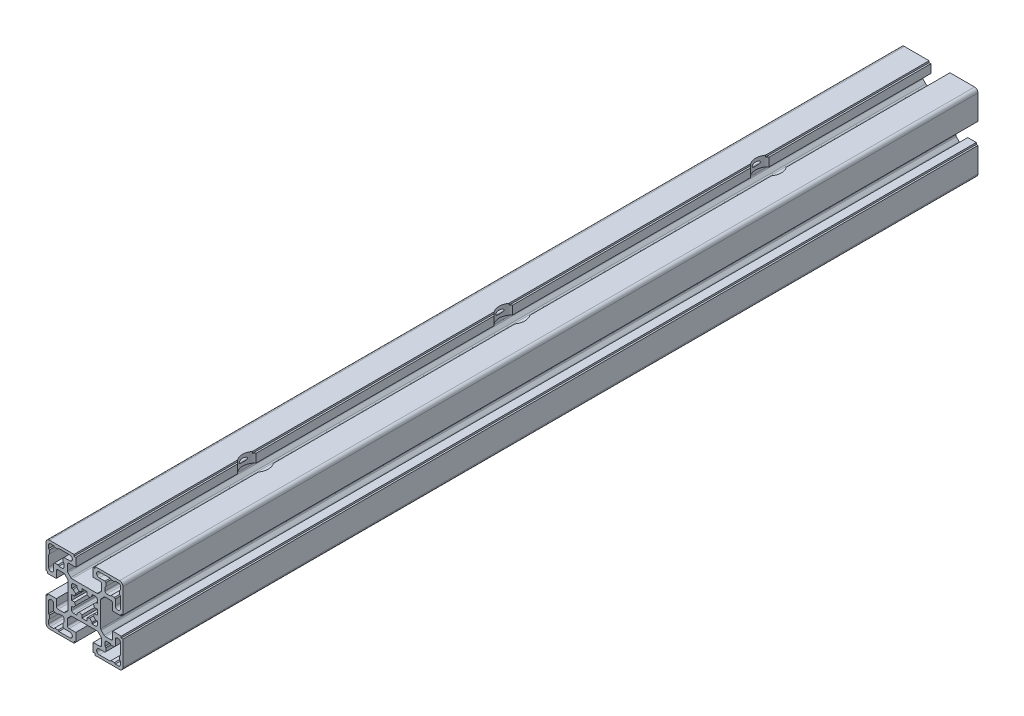
from build123d import *

# Parameters (mm, degrees)
EXTRUDE_1_DEPTH           = 500
HOLE_WIZARD_1_D           = 10
HOLE_WIZARD_1_CBORE_D     = 15
HOLE_WIZARD_1_CBORE_DEPTH = 9


with BuildPart() as part:
    # 草图1 → 拉伸1 (new body)
    with BuildSketch(Plane.XY):
        with BuildLine():
            Line((33.706586033, 40.501982097), (35.388566549, 38.820001582))
            ThreePointArc((35.388566549, 38.820001582), (35.712989897, 38.603228831), (36.09567333, 38.527108363))
            Line((36.09567333, 38.527108363), (39.413692815, 38.527108363))
            ThreePointArc((39.413692815, 38.527108363), (40.120799596, 38.820001582), (40.413692815, 39.527108363))
            Line((40.413692815, 39.527108363), (40.413692815, 43.427108363))
            Line((40.413692815, 43.427108363), (45.413692815, 43.427108363))
            Line((45.413692815, 43.427108363), (45.413692815, 42.427108363))
            Line((45.413692815, 42.427108363), (46.413692815, 42.427108363))
            Line((46.413692815, 42.427108363), (46.413692815, 28.027108363))
            ThreePointArc((46.413692815, 28.027108363), (45.827906377, 26.612894801), (44.413692815, 26.027108363))
            Line((44.413692815, 26.027108363), (30.013692814, 26.027108363))
            Line((30.013692814, 26.027108363), (30.013692814, 27.027108363))
            Line((30.013692814, 27.027108363), (29.013692814, 27.027108363))
            Line((29.013692814, 27.027108363), (29.013692814, 32.027108363))
            Line((29.013692814, 32.027108363), (32.913692814, 32.027108363))
            ThreePointArc((32.913692814, 32.027108363), (33.620799596, 32.320001582), (33.913692814, 33.027108363))
            Line((33.913692814, 33.027108363), (33.913692814, 36.345127848))
            ThreePointArc((33.913692814, 36.345127848), (33.837572347, 36.72781128), (33.620799596, 37.052234629))
            Line((33.620799596, 37.052234629), (31.938819081, 38.734215144))
            ThreePointArc((31.938819081, 38.734215144), (31.614395732, 38.950987895), (31.231712299, 39.027108363))
            Line((31.231712299, 39.027108363), (16.59567333, 39.027108363))
            ThreePointArc((16.59567333, 39.027108363), (16.212989897, 38.950987895), (15.888566548, 38.734215144))
            Line((15.888566548, 38.734215144), (14.206586033, 37.052234629))
            ThreePointArc((14.206586033, 37.052234629), (13.989813282, 36.72781128), (13.913692814, 36.345127848))
            Line((13.913692814, 36.345127848), (13.913692814, 33.027108363))
            ThreePointArc((13.913692814, 33.027108363), (14.206586033, 32.320001582), (14.913692814, 32.027108363))
            Line((14.913692814, 32.027108363), (18.813692815, 32.027108363))
            Line((18.813692815, 32.027108363), (18.813692815, 27.027108363))
            Line((18.813692815, 27.027108363), (17.813692815, 27.027108363))
            Line((17.813692815, 27.027108363), (17.813692815, 26.027108363))
            Line((17.813692815, 26.027108363), (3.413692814, 26.027108363))
            ThreePointArc((3.413692814, 26.027108363), (1.999479252, 26.612894801), (1.413692814, 28.027108363))
            Line((1.413692814, 28.027108363), (1.413692814, 42.427108363))
            Line((1.413692814, 42.427108363), (2.413692814, 42.427108363))
            Line((2.413692814, 42.427108363), (2.413692814, 43.427108363))
            Line((2.413692814, 43.427108363), (7.413692814, 43.427108363))
            Line((7.413692814, 43.427108363), (7.413692814, 39.527108363))
            ThreePointArc((7.413692814, 39.527108363), (7.706586033, 38.820001582), (8.413692814, 38.527108363))
            Line((8.413692814, 38.527108363), (11.731712299, 38.527108363))
            ThreePointArc((11.731712299, 38.527108363), (12.114395732, 38.603228831), (12.43881908, 38.820001582))
            Line((12.43881908, 38.820001582), (14.120799595, 40.501982097))
            ThreePointArc((14.120799595, 40.501982097), (14.337572347, 40.826405446), (14.413692814, 41.209088878))
            Line((14.413692814, 41.209088878), (14.413692814, 55.845127848))
            ThreePointArc((14.413692814, 55.845127848), (14.337572347, 56.22781128), (14.120799595, 56.552234629))
            Line((14.120799595, 56.552234629), (12.43881908, 58.234215144))
            ThreePointArc((12.43881908, 58.234215144), (12.114395732, 58.450987896), (11.731712299, 58.527108363))
            Line((11.731712299, 58.527108363), (8.413692814, 58.527108363))
            ThreePointArc((8.413692814, 58.527108363), (7.706586033, 58.234215144), (7.413692814, 57.527108363))
            Line((7.413692814, 57.527108363), (7.413692814, 53.627108363))
            Line((7.413692814, 53.627108363), (2.413692814, 53.627108363))
            Line((2.413692814, 53.627108363), (2.413692814, 54.627108363))
            Line((2.413692814, 54.627108363), (1.413692814, 54.627108363))
            Line((1.413692814, 54.627108363), (1.413692814, 69.027108363))
            ThreePointArc((1.413692814, 69.027108363), (1.999479252, 70.441321926), (3.413692814, 71.027108363))
            Line((3.413692814, 71.027108363), (17.813692815, 71.027108363))
            Line((17.813692815, 71.027108363), (17.813692815, 70.027108363))
            Line((17.813692815, 70.027108363), (18.813692815, 70.027108363))
            Line((18.813692815, 70.027108363), (18.813692815, 65.027108363))
            Line((18.813692815, 65.027108363), (14.913692814, 65.027108363))
            ThreePointArc((14.913692814, 65.027108363), (14.206586033, 64.734215145), (13.913692814, 64.027108363))
            Line((13.913692814, 64.027108363), (13.913692814, 60.709088878))
            ThreePointArc((13.913692814, 60.709088878), (13.989813282, 60.326405446), (14.206586033, 60.001982097))
            Line((14.206586033, 60.001982097), (15.888566548, 58.320001582))
            ThreePointArc((15.888566548, 58.320001582), (16.212989897, 58.103228831), (16.59567333, 58.027108363))
            Line((16.59567333, 58.027108363), (31.231712299, 58.027108363))
            ThreePointArc((31.231712299, 58.027108363), (31.614395732, 58.103228831), (31.938819081, 58.320001582))
            Line((31.938819081, 58.320001582), (33.620799596, 60.001982097))
            ThreePointArc((33.620799596, 60.001982097), (33.837572347, 60.326405446), (33.913692814, 60.709088878))
            Line((33.913692814, 60.709088878), (33.913692814, 64.027108363))
            ThreePointArc((33.913692814, 64.027108363), (33.620799596, 64.734215145), (32.913692814, 65.027108363))
            Line((32.913692814, 65.027108363), (29.013692814, 65.027108363))
            Line((29.013692814, 65.027108363), (29.013692814, 70.027108363))
            Line((29.013692814, 70.027108363), (30.013692814, 70.027108363))
            Line((30.013692814, 70.027108363), (30.013692814, 71.027108363))
            Line((30.013692814, 71.027108363), (44.413692815, 71.027108363))
            ThreePointArc((44.413692815, 71.027108363), (45.827906377, 70.441321926), (46.413692815, 69.027108363))
            Line((46.413692815, 69.027108363), (46.413692815, 54.627108363))
            Line((46.413692815, 54.627108363), (45.413692815, 54.627108363))
            Line((45.413692815, 54.627108363), (45.413692815, 53.627108363))
            Line((45.413692815, 53.627108363), (40.413692815, 53.627108363))
            Line((40.413692815, 53.627108363), (40.413692815, 57.527108363))
            ThreePointArc((40.413692815, 57.527108363), (40.120799596, 58.234215144), (39.413692815, 58.527108363))
            Line((39.413692815, 58.527108363), (36.09567333, 58.527108363))
            ThreePointArc((36.09567333, 58.527108363), (35.712989897, 58.450987896), (35.388566549, 58.234215144))
            Line((35.388566549, 58.234215144), (33.706586033, 56.552234629))
            ThreePointArc((33.706586033, 56.552234629), (33.489813282, 56.22781128), (33.413692815, 55.845127848))
            Line((33.413692815, 55.845127848), (33.413692815, 41.209088878))
            ThreePointArc((33.413692815, 41.209088878), (33.489813282, 40.826405446), (33.706586033, 40.501982097))
        make_face()
        with BuildLine():
            Line((30.535013158, 44.027108363), (29.082272168, 45.479849354))
            ThreePointArc((29.082272168, 45.479849354), (29.45697001, 46.231007769), (29.723167834, 47.027108363))
            Line((29.723167834, 47.027108363), (31.413692814, 47.027108363))
            Line((31.413692814, 47.027108363), (31.413692814, 50.027108363))
            Line((31.413692814, 50.027108363), (29.723167834, 50.027108363))
            ThreePointArc((29.723167834, 50.027108363), (29.45697001, 50.823208957), (29.082272168, 51.574367373))
            Line((29.082272168, 51.574367373), (30.535013158, 53.027108363))
            Line((30.535013158, 53.027108363), (31.413692814, 53.027108363))
            Line((31.413692814, 53.027108363), (31.413692814, 55.027108363))
            ThreePointArc((31.413692814, 55.027108363), (31.120799596, 55.734215144), (30.413692814, 56.027108363))
            Line((30.413692814, 56.027108363), (28.413692814, 56.027108363))
            Line((28.413692814, 56.027108363), (28.413692814, 55.148428707))
            Line((28.413692814, 55.148428707), (26.960951824, 53.695687716))
            ThreePointArc((26.960951824, 53.695687716), (26.209793409, 54.070385558), (25.413692814, 54.336583382))
            Line((25.413692814, 54.336583382), (25.413692814, 56.027108363))
            Line((25.413692814, 56.027108363), (22.413692814, 56.027108363))
            Line((22.413692814, 56.027108363), (22.413692814, 54.336583382))
            ThreePointArc((22.413692814, 54.336583382), (21.61759222, 54.070385558), (20.866433805, 53.695687716))
            Line((20.866433805, 53.695687716), (19.413692814, 55.148428707))
            Line((19.413692814, 55.148428707), (19.413692814, 56.027108363))
            Line((19.413692814, 56.027108363), (17.413692814, 56.027108363))
            ThreePointArc((17.413692814, 56.027108363), (16.706586033, 55.734215144), (16.413692814, 55.027108363))
            Line((16.413692814, 55.027108363), (16.413692814, 53.027108363))
            Line((16.413692814, 53.027108363), (17.292372471, 53.027108363))
            Line((17.292372471, 53.027108363), (18.745113461, 51.574367373))
            ThreePointArc((18.745113461, 51.574367373), (18.370415619, 50.823208957), (18.104217795, 50.027108363))
            Line((18.104217795, 50.027108363), (16.413692814, 50.027108363))
            Line((16.413692814, 50.027108363), (16.413692814, 47.027108363))
            Line((16.413692814, 47.027108363), (18.104217795, 47.027108363))
            ThreePointArc((18.104217795, 47.027108363), (18.370415619, 46.231007769), (18.745113461, 45.479849354))
            Line((18.745113461, 45.479849354), (17.292372471, 44.027108363))
            Line((17.292372471, 44.027108363), (16.413692814, 44.027108363))
            Line((16.413692814, 44.027108363), (16.413692814, 42.027108363))
            ThreePointArc((16.413692814, 42.027108363), (16.706586033, 41.320001582), (17.413692814, 41.027108363))
            Line((17.413692814, 41.027108363), (19.413692814, 41.027108363))
            Line((19.413692814, 41.027108363), (19.413692814, 41.90578802))
            Line((19.413692814, 41.90578802), (20.866433805, 43.35852901))
            ThreePointArc((20.866433805, 43.35852901), (21.61759222, 42.983831168), (22.413692814, 42.717633344))
            Line((22.413692814, 42.717633344), (22.413692814, 41.027108363))
            Line((22.413692814, 41.027108363), (25.413692814, 41.027108363))
            Line((25.413692814, 41.027108363), (25.413692814, 42.717633344))
            ThreePointArc((25.413692814, 42.717633344), (26.209793409, 42.983831168), (26.960951824, 43.35852901))
            Line((26.960951824, 43.35852901), (28.413692814, 41.90578802))
            Line((28.413692814, 41.90578802), (28.413692814, 41.027108363))
            Line((28.413692814, 41.027108363), (30.413692814, 41.027108363))
            ThreePointArc((30.413692814, 41.027108363), (31.120799596, 41.320001582), (31.413692814, 42.027108363))
            Line((31.413692814, 42.027108363), (31.413692814, 44.027108363))
            Line((31.413692814, 44.027108363), (30.535013158, 44.027108363))
        make_face(mode=Mode.SUBTRACT)
        with BuildLine():
            Line((11.413692814, 66.027108363), (11.913692814, 66.527108364))
            Line((11.913692814, 66.527108364), (15.313692814, 66.527108364))
            ThreePointArc((15.313692814, 66.527108364), (16.813692814, 68.027108363), (15.313692814, 69.527108363))
            Line((15.313692814, 69.527108363), (8.913692815, 69.527108363))
            Line((8.913692815, 69.527108363), (8.413692814, 69.027108363))
            Line((8.413692814, 69.027108363), (6.413692814, 69.027108363))
            Line((6.413692814, 69.027108363), (5.913692814, 69.527108363))
            Line((5.913692814, 69.527108363), (3.913692814, 69.527108363))
            ThreePointArc((3.913692814, 69.527108363), (3.206586033, 69.234215145), (2.913692814, 68.527108363))
            Line((2.913692814, 68.527108363), (2.913692814, 66.527108363))
            Line((2.913692814, 66.527108363), (3.413692814, 66.027108363))
            Line((3.413692814, 66.027108363), (3.413692814, 64.027108363))
            Line((3.413692814, 64.027108363), (2.913692814, 63.527108363))
            Line((2.913692814, 63.527108363), (2.913692814, 57.127108364))
            ThreePointArc((2.913692814, 57.127108364), (4.413692814, 55.627108364), (5.913692814, 57.127108364))
            Line((5.913692814, 57.127108364), (5.913692814, 60.527108363))
            Line((5.913692814, 60.527108363), (6.413692814, 61.027108363))
            Line((6.413692814, 61.027108363), (8.413692814, 61.027108363))
            Line((8.413692814, 61.027108363), (8.913692814, 60.527108363))
            Line((8.913692814, 60.527108363), (10.913692814, 60.527108363))
            ThreePointArc((10.913692814, 60.527108363), (11.620799595, 60.820001582), (11.913692814, 61.527108363))
            Line((11.913692814, 61.527108363), (11.913692814, 63.527108363))
            Line((11.913692814, 63.527108363), (11.413692814, 64.027108363))
            Line((11.413692814, 64.027108363), (11.413692814, 66.027108363))
        make_face(mode=Mode.SUBTRACT)
        with BuildLine():
            Line((11.913692815, 30.527108363), (11.413692814, 31.027108363))
            Line((11.413692814, 31.027108363), (11.413692814, 33.027108363))
            Line((11.413692814, 33.027108363), (11.913692815, 33.527108363))
            Line((11.913692815, 33.527108363), (11.913692815, 35.527108363))
            ThreePointArc((11.913692815, 35.527108363), (11.620799596, 36.234215144), (10.913692815, 36.527108363))
            Line((10.913692815, 36.527108363), (8.913692815, 36.527108363))
            Line((8.913692815, 36.527108363), (8.413692815, 36.027108363))
            Line((8.413692815, 36.027108363), (6.413692814, 36.027108363))
            Line((6.413692814, 36.027108363), (5.913692814, 36.527108363))
            Line((5.913692814, 36.527108363), (5.913692814, 39.927108363))
            ThreePointArc((5.913692814, 39.927108363), (4.413692814, 41.427108363), (2.913692814, 39.927108363))
            Line((2.913692814, 39.927108363), (2.913692814, 33.527108363))
            Line((2.913692814, 33.527108363), (3.413692814, 33.027108363))
            Line((3.413692814, 33.027108363), (3.413692814, 31.027108363))
            Line((3.413692814, 31.027108363), (2.913692814, 30.527108363))
            Line((2.913692814, 30.527108363), (2.913692814, 28.527108363))
            ThreePointArc((2.913692814, 28.527108363), (3.206586033, 27.820001582), (3.913692814, 27.527108363))
            Line((3.913692814, 27.527108363), (5.913692814, 27.527108363))
            Line((5.913692814, 27.527108363), (6.413692814, 28.027108363))
            Line((6.413692814, 28.027108363), (8.413692814, 28.027108363))
            Line((8.413692814, 28.027108363), (8.913692815, 27.527108363))
            Line((8.913692815, 27.527108363), (15.313692814, 27.527108363))
            ThreePointArc((15.313692814, 27.527108363), (16.813692814, 29.027108363), (15.313692814, 30.527108363))
            Line((15.313692814, 30.527108363), (11.913692815, 30.527108363))
        make_face(mode=Mode.SUBTRACT)
        with BuildLine():
            Line((41.913692815, 36.527108363), (41.413692815, 36.027108363))
            Line((41.413692815, 36.027108363), (39.413692815, 36.027108363))
            Line((39.413692815, 36.027108363), (38.913692814, 36.527108363))
            Line((38.913692814, 36.527108363), (36.913692815, 36.527108363))
            ThreePointArc((36.913692815, 36.527108363), (36.206586033, 36.234215145), (35.913692815, 35.527108363))
            Line((35.913692815, 35.527108363), (35.913692815, 33.527108364))
            Line((35.913692815, 33.527108364), (36.413692815, 33.027108363))
            Line((36.413692815, 33.027108363), (36.413692815, 31.027108363))
            Line((36.413692815, 31.027108363), (35.913692815, 30.527108363))
            Line((35.913692815, 30.527108363), (32.513692815, 30.527108363))
            ThreePointArc((32.513692815, 30.527108363), (31.013692815, 29.027108363), (32.513692815, 27.527108363))
            Line((32.513692815, 27.527108363), (38.913692814, 27.527108363))
            Line((38.913692814, 27.527108363), (39.413692814, 28.027108363))
            Line((39.413692814, 28.027108363), (41.413692814, 28.027108363))
            Line((41.413692814, 28.027108363), (41.913692815, 27.527108363))
            Line((41.913692815, 27.527108363), (43.913692815, 27.527108363))
            ThreePointArc((43.913692815, 27.527108363), (44.620799596, 27.820001582), (44.913692815, 28.527108363))
            Line((44.913692815, 28.527108363), (44.913692815, 30.527108363))
            Line((44.913692815, 30.527108363), (44.413692814, 31.027108363))
            Line((44.413692814, 31.027108363), (44.413692814, 33.027108363))
            Line((44.413692814, 33.027108363), (44.913692815, 33.527108364))
            Line((44.913692815, 33.527108364), (44.913692815, 39.927108363))
            ThreePointArc((44.913692815, 39.927108363), (43.413692815, 41.427108363), (41.913692815, 39.927108363))
            Line((41.913692815, 39.927108363), (41.913692815, 36.527108363))
        make_face(mode=Mode.SUBTRACT)
        with BuildLine():
            Line((35.913692815, 66.527108363), (36.413692815, 66.027108363))
            Line((36.413692815, 66.027108363), (36.413692815, 64.027108363))
            Line((36.413692815, 64.027108363), (35.913692815, 63.527108363))
            Line((35.913692815, 63.527108363), (35.913692815, 61.527108363))
            ThreePointArc((35.913692815, 61.527108363), (36.206586033, 60.820001582), (36.913692815, 60.527108363))
            Line((36.913692815, 60.527108363), (38.913692814, 60.527108363))
            Line((38.913692814, 60.527108363), (39.413692815, 61.027108364))
            Line((39.413692815, 61.027108364), (41.413692815, 61.027108364))
            Line((41.413692815, 61.027108364), (41.913692815, 60.527108363))
            Line((41.913692815, 60.527108363), (41.913692815, 57.127108364))
            ThreePointArc((41.913692815, 57.127108364), (43.413692815, 55.627108364), (44.913692815, 57.127108364))
            Line((44.913692815, 57.127108364), (44.913692815, 63.527108363))
            Line((44.913692815, 63.527108363), (44.413692815, 64.027108363))
            Line((44.413692815, 64.027108363), (44.413692815, 66.027108363))
            Line((44.413692815, 66.027108363), (44.913692815, 66.527108363))
            Line((44.913692815, 66.527108363), (44.913692815, 68.527108363))
            ThreePointArc((44.913692815, 68.527108363), (44.620799596, 69.234215145), (43.913692815, 69.527108363))
            Line((43.913692815, 69.527108363), (41.913692815, 69.527108363))
            Line((41.913692815, 69.527108363), (41.413692814, 69.027108363))
            Line((41.413692814, 69.027108363), (39.413692814, 69.027108363))
            Line((39.413692814, 69.027108363), (38.913692814, 69.527108363))
            Line((38.913692814, 69.527108363), (32.513692815, 69.527108363))
            ThreePointArc((32.513692815, 69.527108363), (31.013692815, 68.027108363), (32.513692815, 66.527108363))
            Line((32.513692815, 66.527108363), (35.913692815, 66.527108363))
        make_face(mode=Mode.SUBTRACT)
    extrude(amount=EXTRUDE_1_DEPTH)

    # 打孔尺寸(%根据)内六角圆柱头螺钉的类型1 (through all)
    with Locations(Plane(origin=(0, 71.027108363, 0), x_dir=(1, 0, 0), z_dir=(0, 1, 0))):
        with Locations((23.913692814, -400), (23.913692814, -250), (23.913692814, -100)):
            CounterBoreHole(HOLE_WIZARD_1_D / 2, HOLE_WIZARD_1_CBORE_D / 2, HOLE_WIZARD_1_CBORE_DEPTH)


solid = part.part
